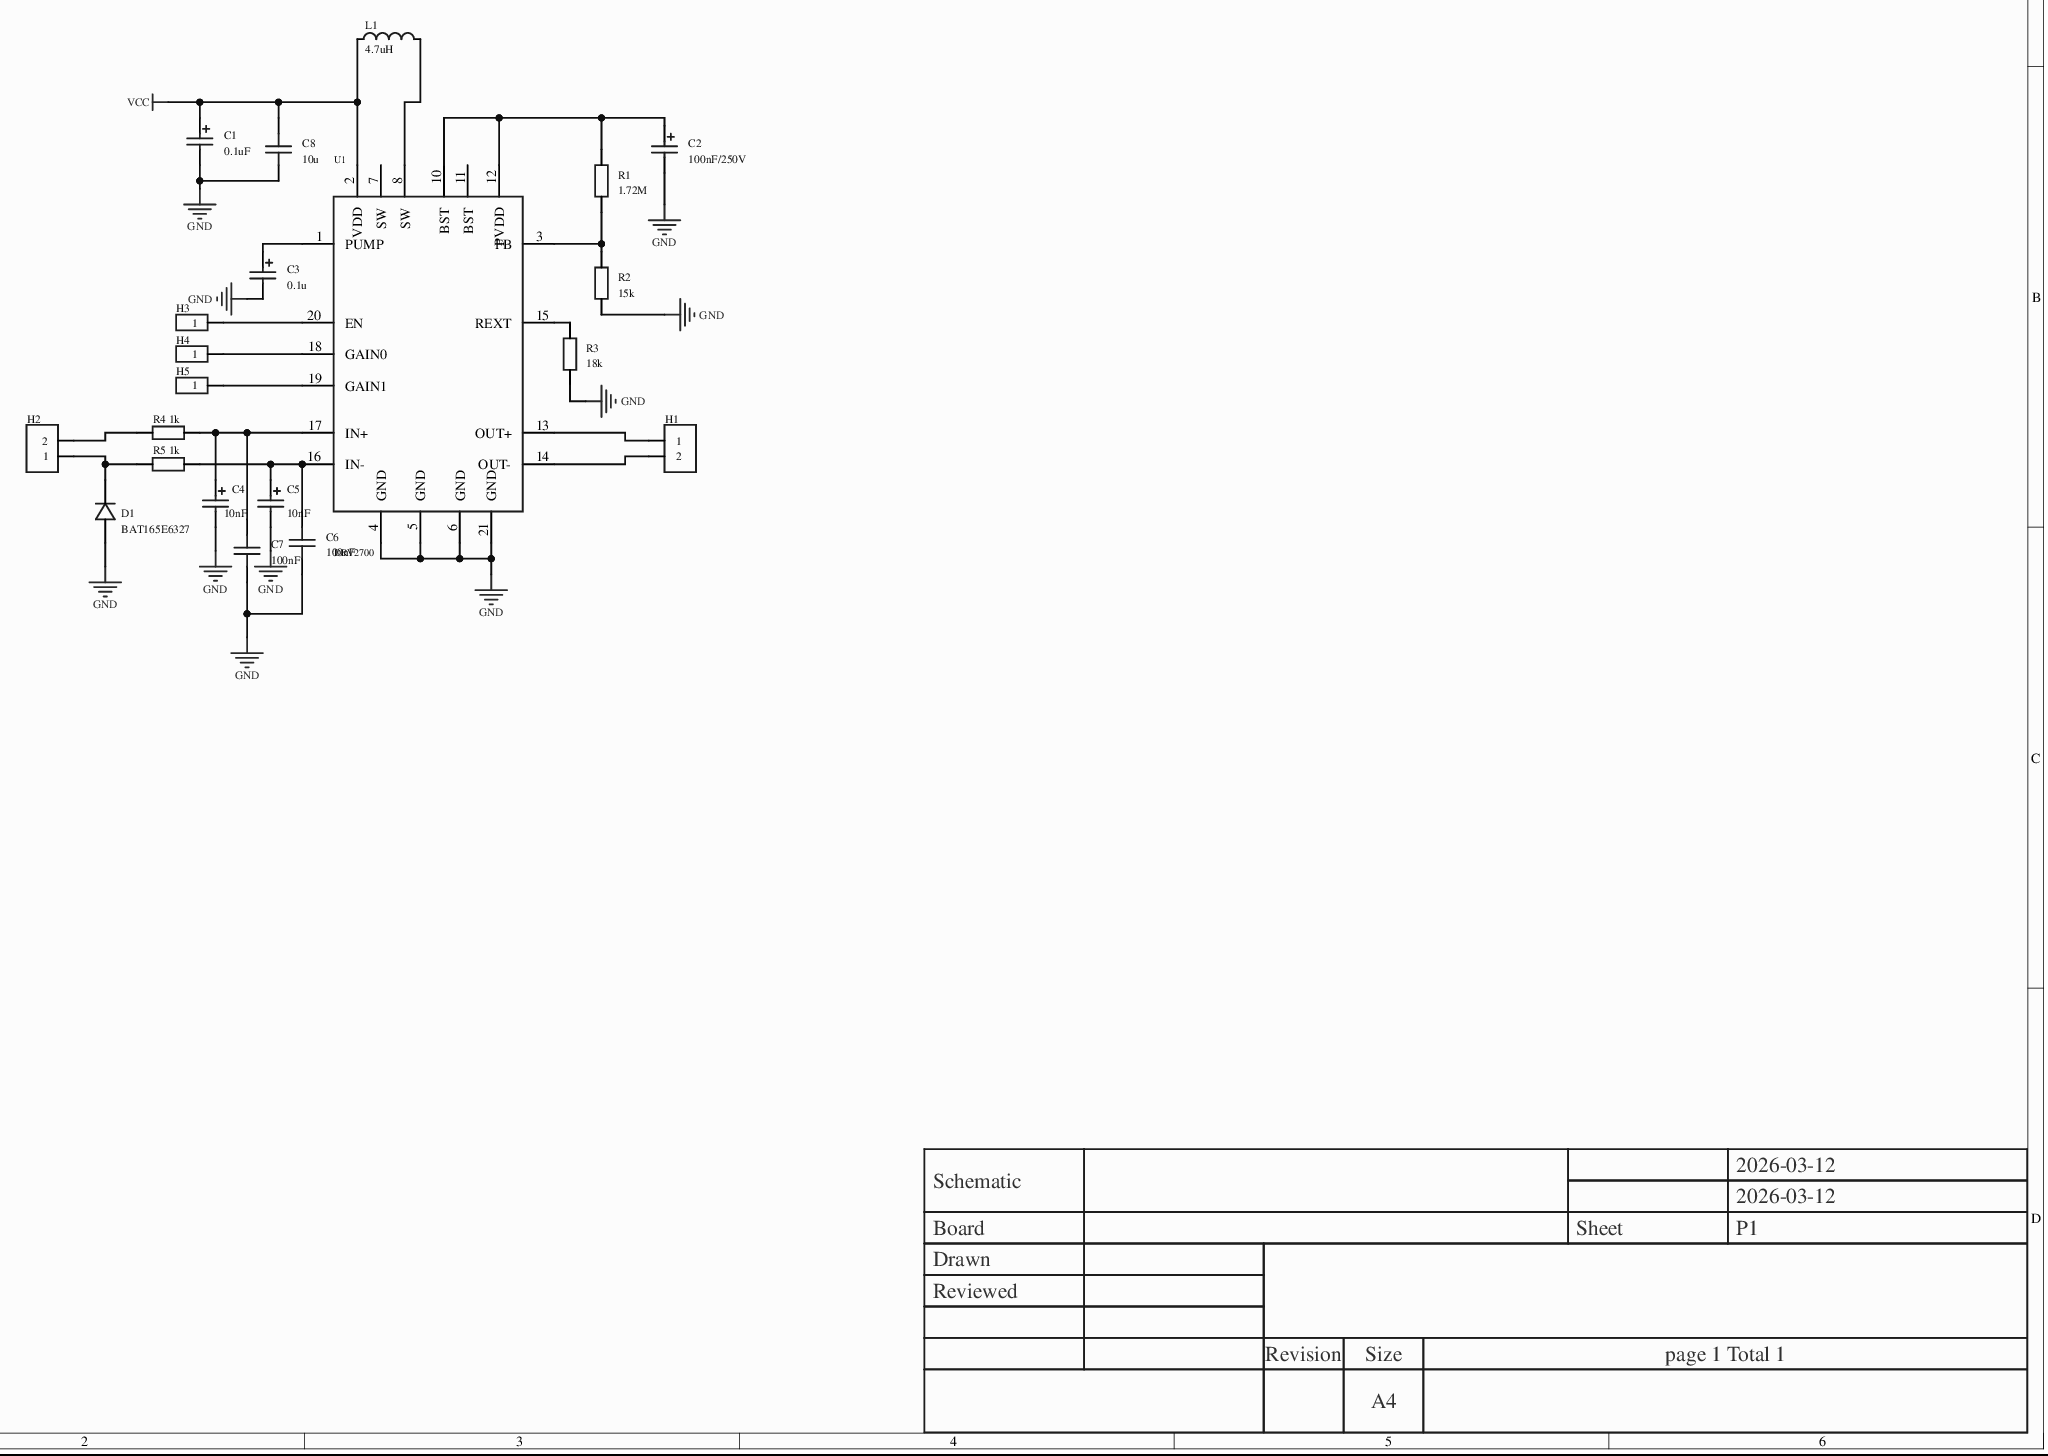
[diagram p0: MISC51337-3.schdoc]
# Altium project MISC51337-2.PrjPcb
1 sheet, 21 parts. Net scope: global (net labels, ports and power ports of the same name join across sheets).
Board file: MISC51337.pcbdoc

## Sheet MISC51337-3.schdoc
size 420 x 297 mm; Version: V1.0; @Project Name: MISC51337; @Update Date: 2026-03-13; @Create Date: 2026-03-13; @Board Name: MISC51337; @Create Time: 20:29:02; @Page Count: 1; @Page No: 1; @Schematic Name: MISC51337; @Update Time: 20:29:02; Size: A4

### Parts
C1  0.1uF  [C_Ele_SMD_3x5.4mm]
C2  100nF/250V  [C_Ele_SMD_3x5.4mm]
C3  0.1u  [C_Ele_SMD_3x5.4mm]
C4  10nF  [C_Ele_SMD_3x5.4mm]
C5  10nF  [C_Ele_SMD_3x5.4mm]
C6  100nF  [C0805]
C7  100nF  [C0805]
C8  10u  [C0805]
D1  BAT165E6327  [SOD-323_L1.8-W1.3-LS2.5-RD]
H1  (no value)  [HDR-TH_2P-P2.54-V-F]
H2  (no value)  [HDR-TH_2P-P2.54-V-F]
H3  (no value)  [HDR-TH_1P-V-M_XKB_X4611WV-01I-C28D40]
H4  (no value)  [HDR-TH_1P-V-M_XKB_X4611WV-01I-C28D40]
H5  (no value)  [HDR-TH_1P-V-M_XKB_X4611WV-01I-C28D40]
L1  4.7uH  [IND-SMD_L4.6-W4.1-A]
R1  1.72M  [Res_1W]
R2  15k  [Res_1W]
R3  18k  [Res_1/4W]
R4  1k  [Res_1/4W]
R5  1k  [Res_1/4W]
U1  DRV2700  [TI-RGP20-2700X2700TP_V]

### Nets
GND: C1.2 C2.2 C3.2 C4.2 C5.2 C6.1 C7.1 C8.1 D1.2(A) R2.1 R3.1 U1.4(GND) U1.5(GND) U1.6(GND) U1.21(GND)
VCC: C1.1 C8.2 L1.1 U1.2(VDD)
NetC2_1: C2.1 R1.2 U1.10(BST) U1.12(PVDD)
NetC3_1: C3.1 U1.1(PUMP)
NetC4_1: C4.1 C7.2 R4.2 U1.17(IN+)
NetC5_1: C5.1 C6.2 R5.2 U1.16(IN-)
NetD1_1: D1.1(C) H2.1 R5.1
NetH1_1: H1.1 U1.13(OUT+)
NetH1_2: H1.2 U1.14(OUT-)
NetH2_2: H2.2 R4.1
NetH3_1: H3.1 U1.20(EN)
NetH4_1: H4.1 U1.18(GAIN0)
NetH5_1: H5.1 U1.19(GAIN1)
NetL1_2: L1.2 U1.8(SW)
NetR1_1: R1.1 R2.2 U1.3(FB)
NetR3_2: R3.2 U1.15(REXT)

Not connected (* = marked no-connect by the designer): U1 7(SW)* 11(BST)*

### Notes on the sheet
- 2026-03-12
- Schematic
- Board
- Sheet
- P1
- Drawn
- Reviewed
- Revision
- Size
- A4
- page 1 Total 1

### Library data of the parts
C1-C5 = C_Ele_SMD_3x5.4mm: Symbol: CAP; AddInBom: yes; ModelId: 0132c3d3fdbf4fd987f710a97e7a5b5d0819f05c4eef4c71ace90d822a990e87; ModelName: CAP-SMD_BD3.0-L3.3-W3.3-H5.3; ModelTransform: 129.9,149.58,209.06,-90,0,0,0,0,0; Device: C_Ele_SMD_3x5.4mm; FootprintName: C_Ele_SMD_3x5.4mm; Supplier Footprint: SMD,3x5.4mm; ConvertToPcb: yes
  C1: Value: 0.1uF
  C2: Value: 100nF/250V
  C3: Value: 0.1u
  C4 C5: Value: 10nF
C6-C8 = CAP_0805: Symbol: Capacitance; ConvertToPcb: yes; ModelId: 1ba041120af144c991958decab20d2410819f05c4eef4c71ace90d822a990e87; ModelName: C0805_L2.0-W1.3-H1.3; ModelTransform: 78.74,51.181,0,0,0,0,0,0.0005,0; Device: CAP_0805; FootprintName: C0805; AddInBom: yes; Supplier Footprint: 0805
  C6 C7: Value: 100nF
  C8: Value: 10u
D1 = BAT165E6327: component BAT165E6327 compon Diode configuration: 1 independent; forward voltage (Vf): 740mV@750mA; DC reverse voltage (Vr): 40V; rectifier current: 750mA;; Manufacturer: Infineon(英飞凌); Symbol: BAT165E6327HTSA1; AddInBom: yes; Reverse Leakage Current (Ir): 50uA@40V; Non-Repetitive Peak Forward Surge Current: 2.5A; ModelId: 7459fe65e23146c0a8d836e46a0add720819f05c4eef4c71ace90d822a990e87; ModelTransform: 104.3305,51.181,0,0,0,0,0,0,0; Device: BAT165E6327; FootprintName: SOD-323_L1.8-W1.3-LS2.5-RD; LCSC Part Name: 电压:40V 电流:750mA; SupplierPart: C151511; ManufacturerPart: BAT165E6327; Supplier Footprint: SOD-323; JLCPCB Part Class: Extended Part; Datasheet: https://item.szlcsc.com/datasheet/BAT165E6327/162851.html; Supplier: LCSC; ConvertToPcb: yes; Diode Configuration: 1 independent; Voltage - Forward(Vf@If): 740mV@750mA; Voltage - DC Reverse(Vr): 40V; Current - Rectified: 750mA; ModelName: SOD-323_L1.8-W1.3-LS2.5-RD
H1 H2 = HDR-F_2.54_1x2P: Symbol: Header-Female-2.54_1x2; ConvertToPcb: yes; ModelId: a9450ef445564560a104363b9aacde4e0819f05c4eef4c71ace90d822a990e87; ModelName: HDR-TH_2P-P2.54-F-LI-1X2P; ModelTransform: 215.7476,98.425,0,0,0,0,0,0,-129.921; Device: HDR-F_2.54_1x2P; FootprintName: HDR-TH_2P-P2.54-V-F; AddInBom: yes; SupplierPart: C49661; Supplier Footprint: 插件
H3-H5 = HDR-M_2.54_1x1P: Symbol: HDR_1x1; ConvertToPcb: yes; ModelId: 95857080d3cc4057a19a22ccce05e1710819f05c4eef4c71ace90d822a990e87; ModelTransform: 78.74,79.1337,0,0,0,0,0,0,-110.236; Device: HDR-M_2.54_1x1P; FootprintName: HDR-TH_1P-V-M_XKB_X4611WV-01I-C28D40; AddInBom: yes; SupplierPart: C81276; Supplier Footprint: 插件; JLCPCB Part Class: Extended Part; ModelName: HDR-TH_1P-V-M_XKB_X4611WV-01I-C28D40
L1 = SRG0420-4R7-M: component SRG0420-4R7-M comp Inductance: 4.7uH; tolerance: ±20%; rated current: 3A; saturation current (Isat): 3.5A; type: molded inductor;; Manufacturer: JIERR(捷而瑞); AddInBom: yes; DC Resistance(DCR): 105mΩ; ModelId: 3b00517e351145dc8b8e2e52a7e5ed2c0819f05c4eef4c71ace90d822a990e87; ModelName: IND-SMD_L4.6-W4.1-H1.5; ModelTransform: 181.102,161.417,0,0,0,0,0,0,0; Device: SRG0420-4R7-M; Symbol: SRG0420-4R7-M; FootprintName: IND-SMD_L4.6-W4.1-A; LCSC Part Name: 4.7μH ±20% 3.5A; SupplierPart: C53462918; ManufacturerPart: SRG0420-4R7-M; Supplier Footprint: SMD,4.6x4.1mm; JLCPCB Part Class: Extended Part; Datasheet: https://item.szlcsc.com/datasheet/SRG0420-4R7-M/56628163.html; Supplier: LCSC; ConvertToPcb: yes; Value: 4.7uH; Tolerance: ±20%; Current Rating: 3A; Current - Saturation(Isat): 3.5A; Type: Molded inductor
R1-R5 = Res_AXIAL-1W: Symbol: Resistor; ConvertToPcb: yes; ModelId: f1f7cfb3d56f4763951150e77c261d090819f05c4eef4c71ace90d822a990e87; ModelName: RES-TH_BD4.5-L11.5-P15.50-D0.8; ModelTransform: 641.71,177.16,374,0,0,0,0,0,-190; Device: Res_AXIAL-1W; AddInBom: yes; Supplier Footprint: 轴向引线
  R1: Value: 1.72M; FootprintName: Res_1W
  R2: Value: 15k; FootprintName: Res_1W
  R3: Value: 18k; FootprintName: Res_1/4W
  R4 R5: Value: 1k; FootprintName: Res_1/4W
U1 = DRV2700: Device: DRV2700; Symbol: DRV2700; FootprintName: TI-RGP20-2700X2700TP_V